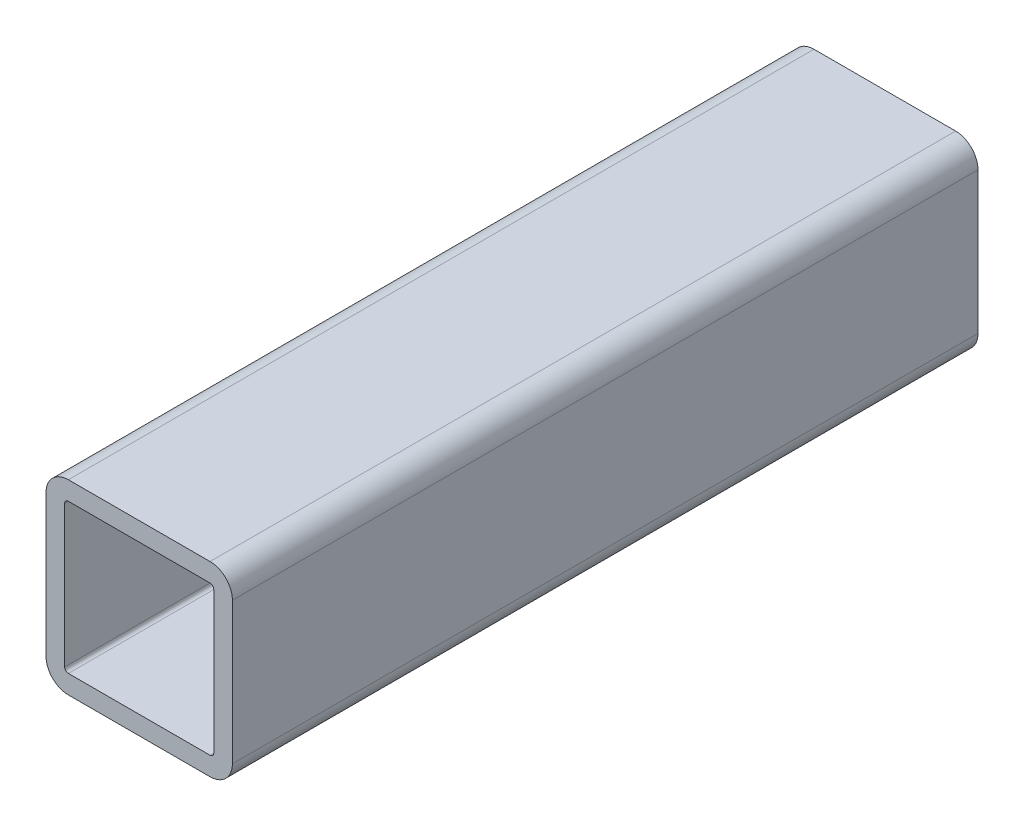
SolidWorks part; units mm, degrees
material "Q235B"
ref_plane "Front Plane" through (0, 0, 0) normal (0, 0, 1) x (1, 0, 0)
ref_plane "Top Plane" through (0, 0, 0) normal (0, 1, 0) x (1, 0, 0)
ref_plane "Right Plane" through (0, 0, 0) normal (1, 0, 0) x (0, 0, -1)
sketch "Sketch1" plane through (0, 0, 0) normal (0, 0, 1) x (1, 0, 0)
  line L0 (6, 45) -> (44, 45)
  line L1 (6, 0) -> (44, 0)
  line L2 (0, 6) -> (0, 44)
  line L3 (6, 50) -> (44, 50)
  line L4 (50, 6) -> (50, 44)
  line L5 (45, 6) -> (45, 44)
  line L6 (6, 5) -> (44, 5)
  line L7 (5, 6) -> (5, 44)
  arc A0 (6, 0) -> (0, 6) centre (6, 6) cw
  arc A1 (44, 0) -> (50, 6) centre (44, 6) ccw
  arc A2 (44, 50) -> (50, 44) centre (44, 44) cw
  arc A3 (0, 44) -> (6, 50) centre (6, 44) cw
  arc A4 (5, 44) -> (6, 45) centre (6, 44) cw
  arc A5 (44, 45) -> (45, 44) centre (44, 44) cw
  arc A6 (44, 5) -> (45, 6) centre (44, 6) ccw
  arc A7 (6, 5) -> (5, 6) centre (6, 6) cw
  point P7 (0, 0)
  point P12 (50, 50)
  point P15 (0, 50)
  dimension "D3" = 6
  dimension "D1" = 50
  dimension "D2" = 50
  dimension "D4" = 5
extrude "Boss-Extrude1" add sketch "Sketch1" along normal blind 200
